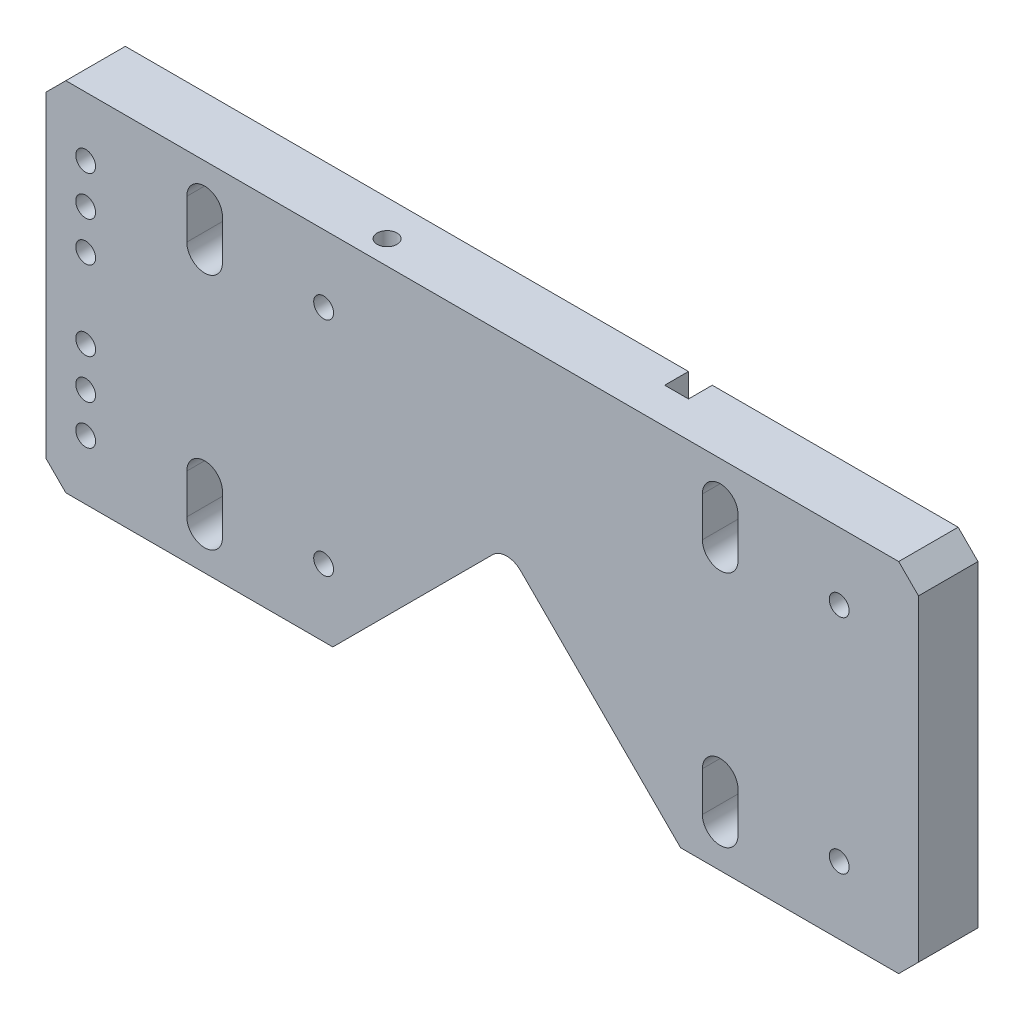
from build123d import *

# Parameters (mm, degrees)
SKETCH1_W             = 220
SKETCH1_H             = 90
BOSS_EXTRUDE1_DEPTH   = 15
M6_TAPPED_HOLE1_D     = 5
M6_TAPPED_HOLE1_DEPTH = 15
M6_TAPPED_HOLE1_TIP   = 1.502151548
CUT_EXTRUDE1_DEPTH    = 239.170107276
CUT_EXTRUDE2_DEPTH    = 239.170107276
M6_TAPPED_HOLE2_D     = 5
M6_TAPPED_HOLE2_DEPTH = 15
M6_TAPPED_HOLE2_TIP   = 1.502151548
CHAMFER1_SIZE         = 5
FILLET1_R             = 5
CUT_EXTRUDE3_DEPTH    = 6
SKETCH11_R            = 2.5
CUT_EXTRUDE4_DEPTH    = 239.170107276


with BuildPart() as part:
    # Sketch1 → Boss-Extrude1 (new body)
    with BuildSketch(Plane.XY):
        with Locations((110, 45)):
            Rectangle(SKETCH1_W, SKETCH1_H)
    extrude(amount=BOSS_EXTRUDE1_DEPTH)

    # M6 Tapped Hole1
    with Locations(Plane.XY.offset(15)):
        with Locations((70, 73), (70, 17), (200, 73), (200, 17)):
            Hole(M6_TAPPED_HOLE1_D / 2, depth=M6_TAPPED_HOLE1_DEPTH)
            with Locations((0, 0, -(M6_TAPPED_HOLE1_DEPTH + M6_TAPPED_HOLE1_TIP / 2))):  # 118° drill point
                Cone(0, M6_TAPPED_HOLE1_D / 2, M6_TAPPED_HOLE1_TIP, mode=Mode.SUBTRACT)

    # Sketch4 → Cut-Extrude1 (cut, through all)
    with BuildSketch(Plane.XY.offset(15)):
        with BuildLine():
            Line((44.5, 80), (44.5, 70))
            ThreePointArc((44.5, 70), (40, 65.5), (35.5, 70))
            Line((35.5, 70), (35.5, 80))
            ThreePointArc((35.5, 80), (40, 84.5), (44.5, 80))
        make_face()
        with BuildLine():
            Line((44.5, 20), (44.5, 10))
            ThreePointArc((44.5, 10), (40, 5.5), (35.5, 10))
            Line((35.5, 10), (35.5, 20))
            ThreePointArc((35.5, 20), (40, 24.5), (44.5, 20))
        make_face()
        with BuildLine():
            Line((174.5, 80), (174.5, 70))
            ThreePointArc((174.5, 70), (170, 65.5), (165.5, 70))
            Line((165.5, 70), (165.5, 80))
            ThreePointArc((165.5, 80), (170, 84.5), (174.5, 80))
        make_face()
        with BuildLine():
            Line((174.5, 20), (174.5, 10))
            ThreePointArc((174.5, 10), (170, 5.5), (165.5, 10))
            Line((165.5, 10), (165.5, 20))
            ThreePointArc((165.5, 20), (170, 24.5), (174.5, 20))
        make_face()
    extrude(amount=-CUT_EXTRUDE1_DEPTH, mode=Mode.SUBTRACT)

    # Sketch5 → Cut-Extrude2 (cut, through all)
    with BuildSketch(Plane.XY.offset(15)):
        Polygon((72.318759133, 0), (116.159379566, 43.840620434), (160, 0), (116.159379566, -43.840620434), align=None)
    extrude(amount=-CUT_EXTRUDE2_DEPTH, mode=Mode.SUBTRACT)

    # M6 Tapped Hole2
    with Locations(Plane(origin=(0, 90, 0), x_dir=(1, 0, 0), z_dir=(0, 1, 0))):
        with Locations((80, -9)):
            Hole(M6_TAPPED_HOLE2_D / 2, depth=M6_TAPPED_HOLE2_DEPTH)
            with Locations((0, 0, -(M6_TAPPED_HOLE2_DEPTH + M6_TAPPED_HOLE2_TIP / 2))):  # 118° drill point
                Cone(0, M6_TAPPED_HOLE2_D / 2, M6_TAPPED_HOLE2_TIP, mode=Mode.SUBTRACT)

    # Chamfer1
    chamfer1_edges = [part.edges().sort_by_distance(p)[0] for p in [
        (0, 90, 7.5),
        (220, 90, 7.5),
        (220, 0, 7.5),
        (0, 0, 7.5),
    ]]
    chamfer(chamfer1_edges, length=CHAMFER1_SIZE)

    # Fillet1
    fillet1_edges = [part.edges().sort_by_distance(p)[0] for p in [
        (116.159379566, 43.840620434, 7.5),
    ]]
    fillet(fillet1_edges, radius=FILLET1_R)

    # Sketch10 → Cut-Extrude3 (cut)
    with BuildSketch(Plane(origin=(0, 0, 0), x_dir=(-1, 0, 0), z_dir=(0, 0, -1))):
        with BuildLine():
            Line((-153, 0), (-153, 90))
            ThreePointArc((-153, 90), (-150, 93), (-147, 90))
            Line((-147, 90), (-147, 0))
            ThreePointArc((-147, 0), (-150, -3), (-153, 0))
        make_face()
    extrude(amount=-CUT_EXTRUDE3_DEPTH, mode=Mode.SUBTRACT)

    # Sketch11 → Cut-Extrude4 (cut, through all)
    with BuildSketch(Plane.XY.offset(15)):
        with Locations((10, 55)):
            Circle(SKETCH11_R)
        with Locations((10, 35)):
            Circle(SKETCH11_R)
        with Locations((10, 25)):
            Circle(SKETCH11_R)
        with Locations((10, 65)):
            Circle(SKETCH11_R)
        with Locations((10, 75)):
            Circle(SKETCH11_R)
        with Locations((10, 15)):
            Circle(SKETCH11_R)
    extrude(amount=-CUT_EXTRUDE4_DEPTH, mode=Mode.SUBTRACT)


solid = part.part
